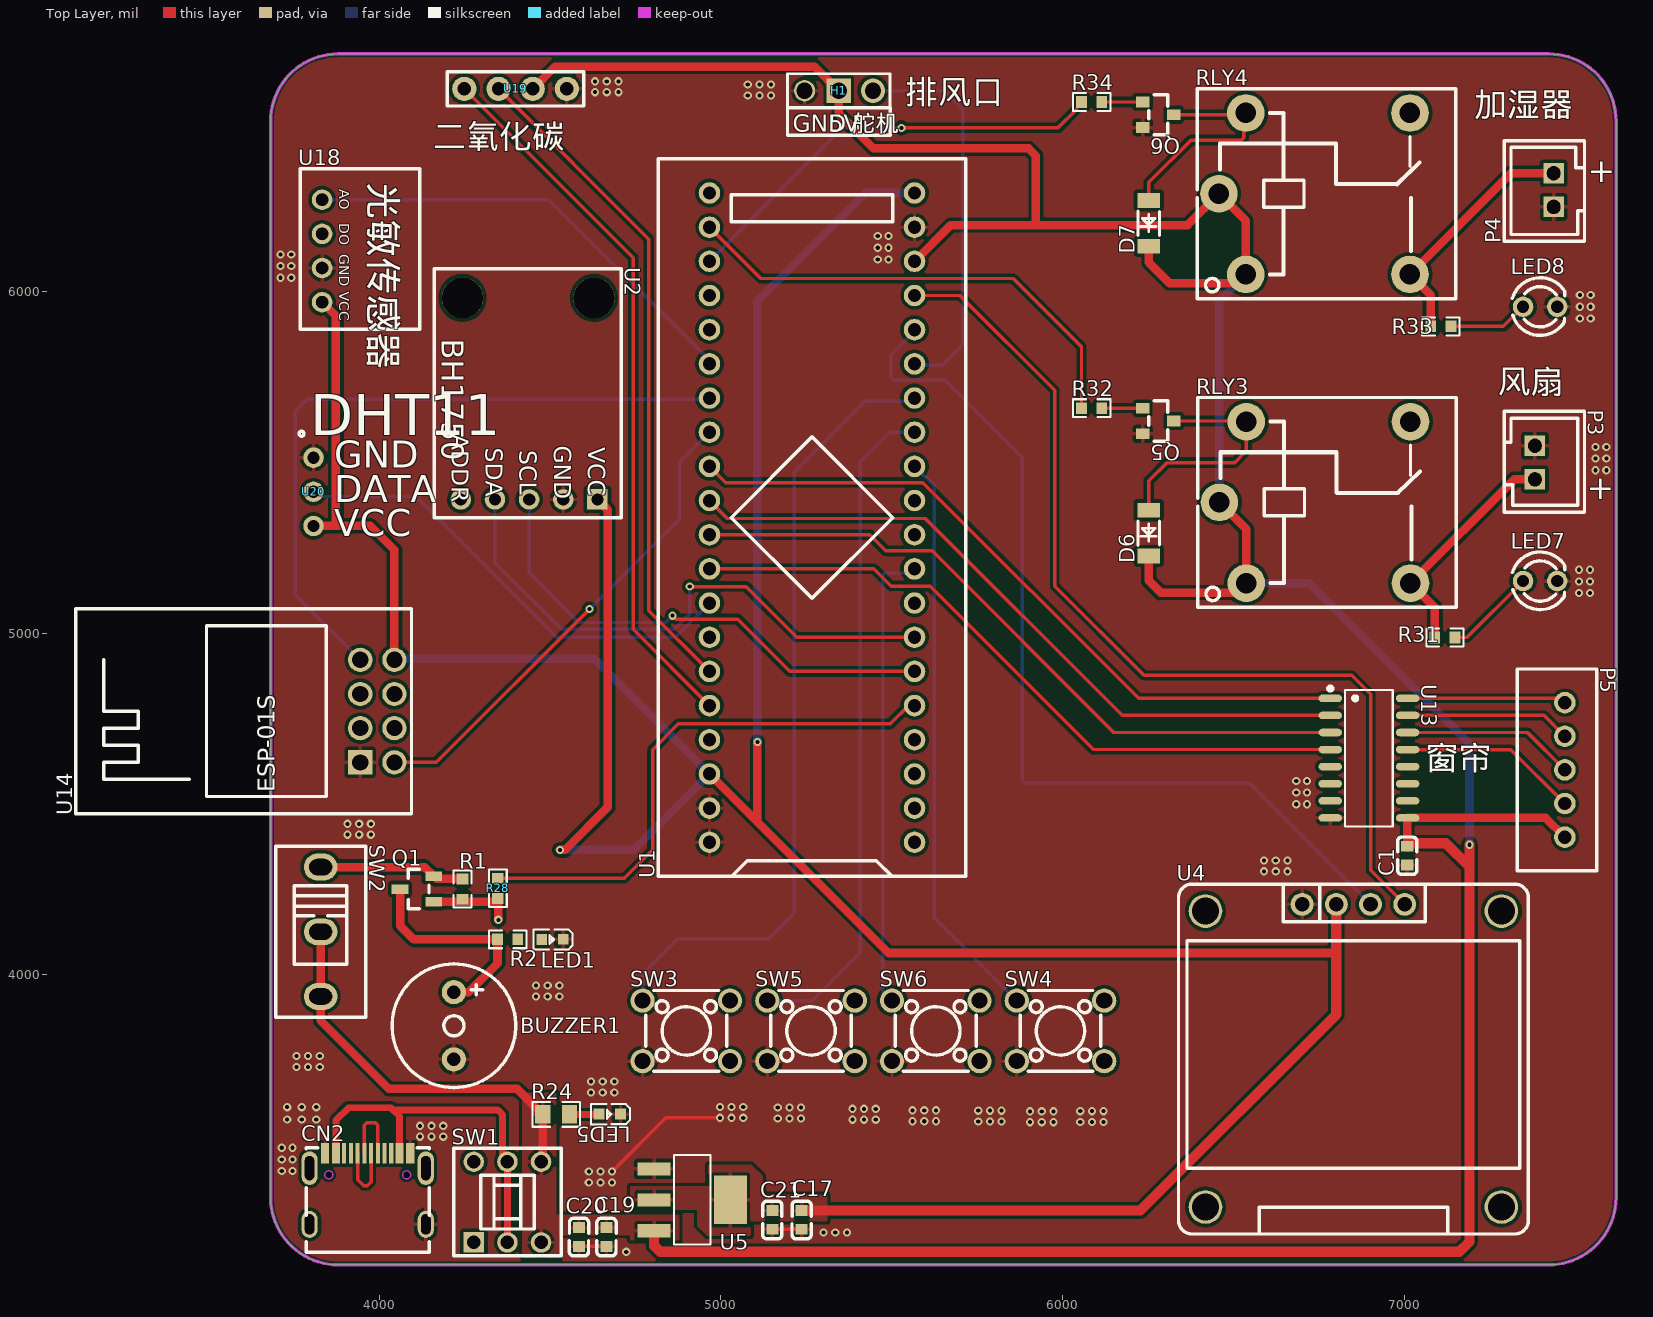
[diagram p0: Top Layer view]
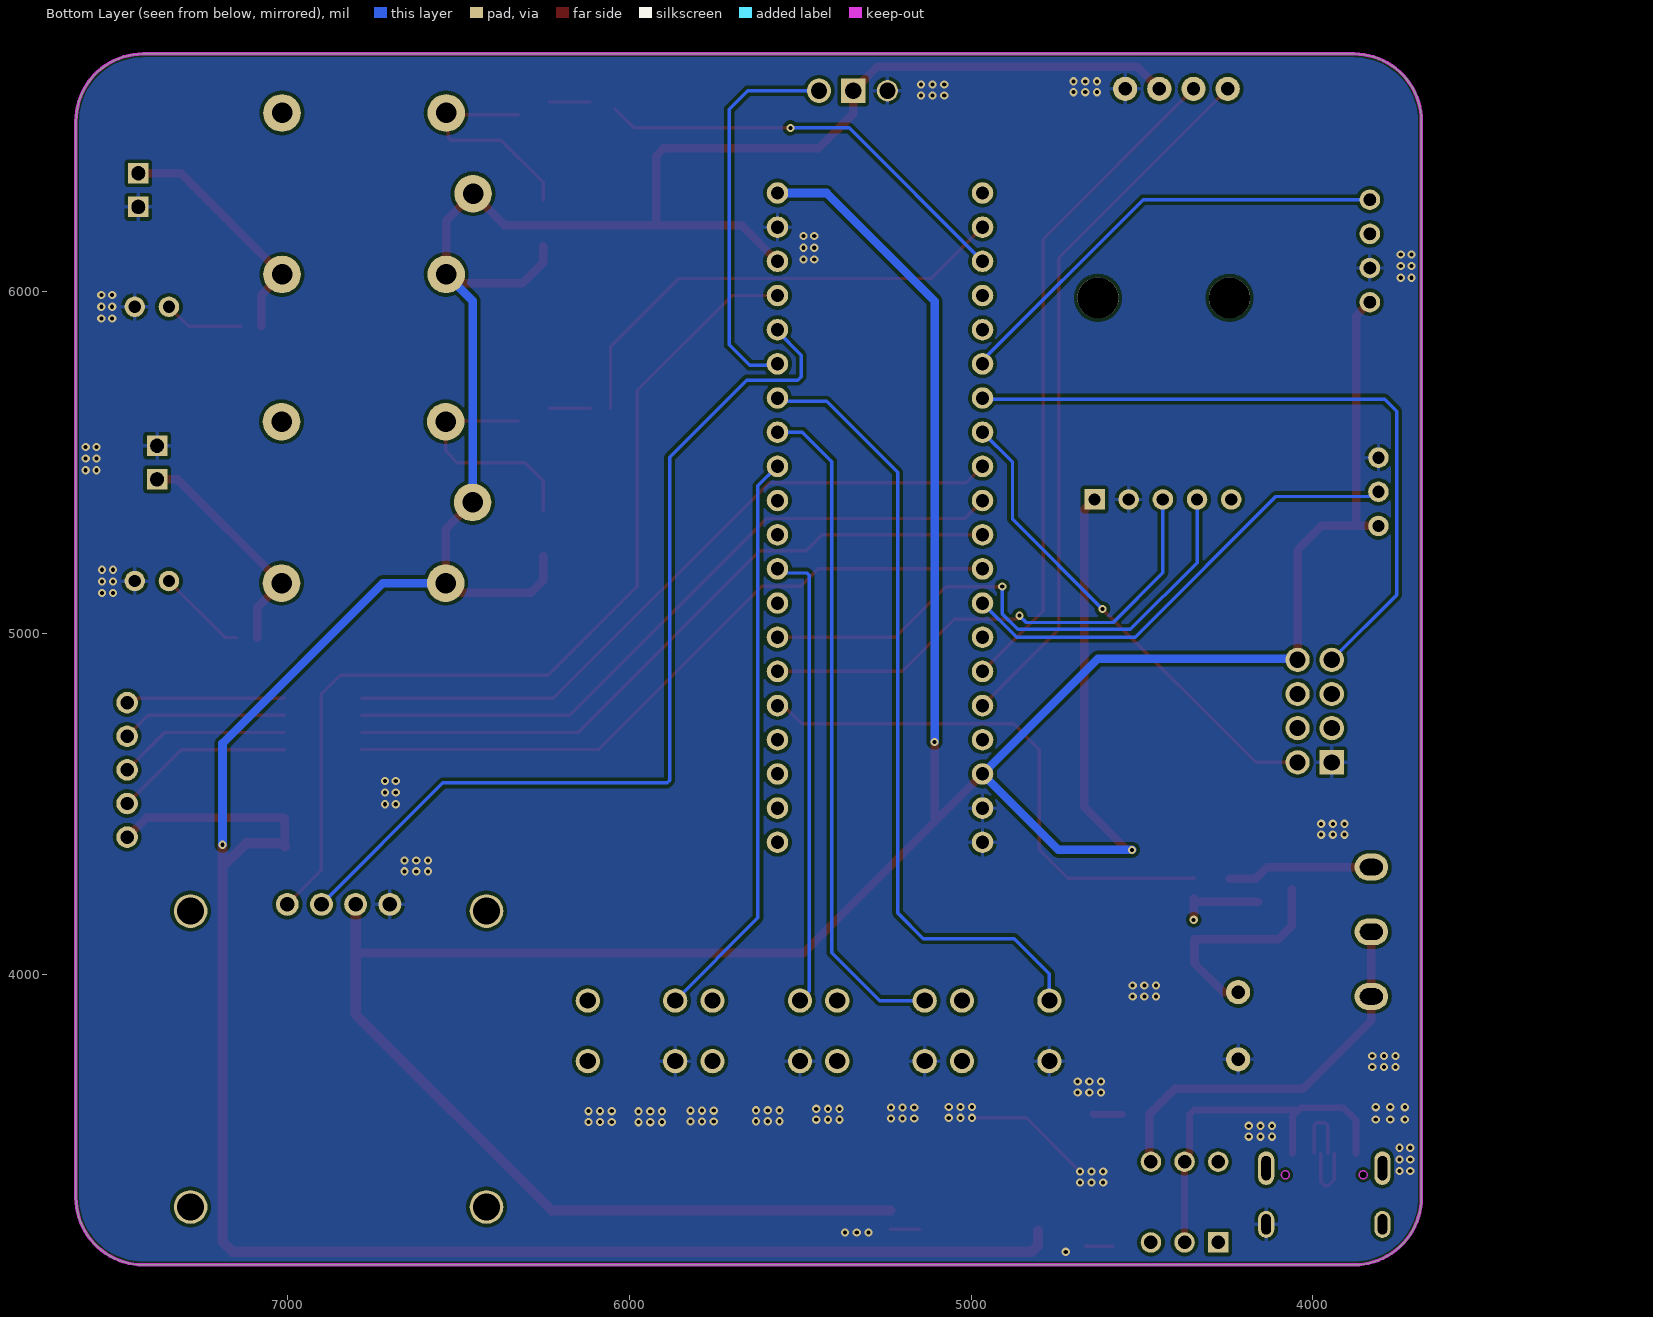
[diagram p1: Bottom Layer view, seen from below]
# Altium PCB MISC51844.pcbdoc
Units mil, origin at the board's own origin, x right, y up, seen from the top; angles counter-clockwise.
Board outline 3937.01 x 3543.31 mil, 2 copper layers (Top Layer, Bottom Layer), stack 62.206 mil thick; 45 components, 47 nets, 206 pads, 156 vias.

## Layer stack, top to bottom
Top Solder Mask Layer: solder mask 0.394, Dk 3.3
Top Layer: signal copper 1.379
Dielectric1: surface 59.449, FR4, Dk 4.5
Bottom Layer: signal copper 1.378
Bottom Solder Mask Layer: solder mask 0.394, Dk 3.3

## Board outline
3879.19,6694.72 ccw(c3879.19,6497.87) 3682.34,6497.87 3682.34,3348.26 ccw(c3879.19,3348.26) 3879.19,3151.41 7422.5,3151.41 ccw(c7422.5,3348.26) 7619.35,3348.26 7619.35,6497.87 ccw(c7422.5,6497.87) 7422.5,6694.72 3879.19,6694.72

## Design rules (kind name [scope] priority, off if disabled: settings)
BoardOutlineClearance copperThickness2oz_1 [All] p2 off: genericclearance=7.99 ignorepadtopadclearanceinfootprint=FALSE except(0: Arc-SplitContinuation Track-SplitContinuation SMDPad-SplitContinuation THPad-SplitContinuation Via-SplitContinuation Fill-SplitContinuation Region-SplitContinuation Poly-SplitContinuation Text-SplitContinuation Hole-SplitContinuation; 5.98: Arc-CutoutEdge SMDPad-CutoutEdge THPad-CutoutEdge Via-CutoutEdge Fill-CutoutEdge Region-CutoutEdge Text-CutoutEdge; 6.93: Hole-OutlineEdge Hole-CutoutEdge; 10: Poly-OutlineEdge Poly-CutoutEdge; 11.81: Arc-OutlineEdge Track-OutlineEdge SMDPad-OutlineEdge THPad-OutlineEdge Via-OutlineEdge Fill-OutlineEdge Region-OutlineEdge Text-OutlineEdge Track-CutoutEdge)
BoardOutlineClearance copperThickness1oz_1 [All] p4: genericclearance=4.02 ignorepadtopadclearanceinfootprint=FALSE except(0: Arc-SplitContinuation Track-SplitContinuation SMDPad-SplitContinuation THPad-SplitContinuation Via-SplitContinuation Fill-SplitContinuation Region-SplitContinuation Poly-SplitContinuation Text-SplitContinuation Hole-SplitContinuation; 6: SMDPad-CutoutEdge THPad-CutoutEdge Via-CutoutEdge Fill-CutoutEdge Region-CutoutEdge Text-CutoutEdge; 6.93: Hole-OutlineEdge Hole-CutoutEdge; 10: Poly-OutlineEdge Poly-CutoutEdge; 11.8: Arc-OutlineEdge Track-OutlineEdge SMDPad-OutlineEdge THPad-OutlineEdge Via-OutlineEdge Fill-OutlineEdge Region-OutlineEdge Text-OutlineEdge; 11.81: Arc-CutoutEdge Track-CutoutEdge)
Clearance copperThickness2oz [All] p1 off: gap=7.99 ignorepadtopadclearanceinfootprint=FALSE except(5.98: SMDPad-Track SMDPad-SMDPad THPad-Track SMDPad-THPad THPad-THPad Track-Via SMDPad-Via THPad-Via Via-Via Fill-Track Region-Track Fill-SMDPad Region-SMDPad Fill-THPad Region-THPad Fill-Via Region-Via Fill-Fill Fill-Region Region-Region Arc-Track Arc-SMDPad Arc-THPad Arc-Via Fill-Arc Region-Arc Arc-Arc Text-Track SMDPad-Text Text-THPad Text-Via Fill-Text Region-Text Arc-Text Text-Text; 6.93: Hole-Track Hole-SMDPad Hole-THPad Hole-Via Fill-Hole Region-Hole Hole-Arc Hole-Text; 10: Poly-Track Poly-SMDPad Poly-THPad Poly-Via Poly-Fill Poly-Region Poly-Poly Poly-Arc Poly-Text Poly-Hole)
Clearance copperThickness1oz [All] p3: gap=4.02 ignorepadtopadclearanceinfootprint=FALSE except(5.98: SMDPad-Track SMDPad-SMDPad THPad-Track SMDPad-THPad THPad-THPad Track-Via SMDPad-Via THPad-Via Via-Via Fill-Track Region-Track Fill-SMDPad Region-SMDPad Fill-THPad Region-THPad Fill-Via Region-Via Fill-Fill Fill-Region Region-Region; 6: Arc-Track Arc-SMDPad Arc-THPad Arc-Via Fill-Arc Region-Arc Arc-Arc Text-Track SMDPad-Text Text-THPad Text-Via Fill-Text Region-Text Arc-Text Text-Text; 6.93: Hole-Track Hole-SMDPad Hole-THPad Hole-Via Fill-Hole Region-Hole Hole-Arc Hole-Text; 10: Poly-Track Poly-SMDPad Poly-THPad Poly-Via Poly-Fill Poly-Region Poly-Poly Poly-Arc Poly-Text Poly-Hole)
DiffPairsRouting differentialPair [All] p1: maxlimit=6 minlimit=6 mostfreqgap=6 toplayer_minwidth=5 toplayer_prefwidth=10 toplayer_maxwidth=100 toplayer_mingap=6 toplayer_prefgap=6 toplayer_maxgap=6 bottomlayer_minwidth=5 bottomlayer_prefwidth=10 bottomlayer_maxwidth=100 bottomlayer_mingap=6 bottomlayer_prefgap=6 bottomlayer_maxgap=6 maxuncoupledlength=10
HoleToHoleClearance otherClearance [All] p1: gap=11.81 allowstackedmicrovias=TRUE
Length netLength [All] p1: minlimit=0 maxlimit=0
MatchedLengths netLengthTolerance [All] p1: tolerance=1000
PasteMaskExpansion pasteMaskExpansion [All] p1: expansion=0
PlaneConnect innerPlane [All] p1: planeconnectstyle=Relief reliefexpansion=20 reliefentries=4 reliefconductorwidth=10 reliefairgap=10
PolygonConnect copperRegion [All] p1: connectstyle=Relief reliefconductorwidth=10 reliefentries=4 polygonreliefangle="90 Angle" airgapwidth=10 via.connectstyle=Relief via.reliefconductorwidth=10 via.reliefentries=4 via.polygonreliefangle="90 Angle" via.airgapwidth=10
RoutingVias viaSize [All] p1: holewidth=12.01 width=24.02 viastyle="Through Hole" minholewidth=11.81 minwidth=19.68 maxholewidth=248.03 maxwidth=393.7
SolderMaskExpansion solderMaskExpansion [IsVia] p1: expansion=-1000 istentingtop=TRUE
SolderMaskExpansion solderMaskExpansion [All] p2: expansion=2 istentingtop=FALSE
Width copperThickness2oz_2 [All] p1 off: maxlimit=100 minlimit=8 preferedwidth=10
Width copperThickness1oz_2 [All] p2: maxlimit=100 minlimit=5 preferedwidth=10

## Components (designator, comment, footprint, x,y, rotation, side; value= is the part's Value field where it differs from the comment)
BUZZER1 "HNB09A03" BUZ-TH_BD9.0-P5.00-D0.6-FD 4218.56,3850.88 r270 top
C1 "47pf" C0603#1 7008.29,4348.46 r90 top
C17 "100n" C0603#2 5236.12,3282.62 r90 top
C19 "100n" C0603#2 4665.04,3232.75 r90 top
C20 "10u" C0603#2 4584.63,3232.75 r90 top
C21 "22u" C0603#2 5150.42,3282.62 r90 top
CN2 "USB-TYPEC" USB-C-SMD_MC-307 3966.22,3373.55 r0 top
D6 "LL4148" LL-34_L3.5-W1.5-RD 6251.77,5292.56 r90 top
D7 "LL4148" LL-34_L3.5-W1.5-RD 6251.77,6198.97 r90 top
H1 "舵机模块" 舵机模块 5344.81,6586.97 r0 top
LED1 "" LED_0603 4504.75,4103.27 r180 top
LED5 "" LED_0603 4672.56,3592.05 r180 top
LED7 "" LED_TH-3mm 7397.24,5152.23 r0 top
LED8 "" LED_TH-3mm 7397.24,5954.86 r0 top
P3 "XH2.54直插座-2P" CONN-TH_XH2.54-2P 7381.88,5498.97 r270 top
P4 "XH2.54直插座-2P" CONN-TH_XH2.54-2P 7436.88,6296.23 r90 top
P5 "" CONN-TH_XH2.54-5P 7469.51,4599.63 r270 top
Q1 "" S8550P_SOT 4108.56,4250.88 r0 top
Q5 "" S8050_SOT-23 6279.53,5625.55 r180 top
Q6 "" S8050_SOT-23 6279.53,6521.7 r180 top
R1 "10k" R0603 4243.56,4250.88 r270 top
R2 "1k" R0603 4375.75,4103.67 r180 top
R24 "4.7k" R0805 4517.71,3591.37 r0 top
R28 "1k" R0603 4347.14,4252.97 r270 top
R31 "3.3k" R0603 7118.6,4987.04 r0 top
R32 "1k" R0603 6084.73,5658.26 r0 top
R33 "3.3k" R0603 7106.6,5897.3 r0 top
R34 "1k" R0603 6084.73,6554.14 r0 top
RLY3 "SRD-05VDC-SL-C" RELAY-TH_SRD-XXVDC-XL-C 6738.22,5382.36 r0 top
RLY4 "SRD-05VDC-SL-C" RELAY-TH_SRD-XXVDC-XL-C 6736.75,6285.76 r0 top
SW1 "K8-8081D-NNW" SW-TH_6P-L8.0-W8.0-P2.50 4375.18,3334.76 r0 top
SW2 "XY-SS12D10L3" SW-TH_3P-L12.7-W6.7_XY-SS12D10LXX 3828.56,4125.88 r270 top
SW3 "" SW-TH_4P-L6.0-W6.0-P4.50-LS6.5 4898.56,3835.88 r0 top
SW4 "" SW-TH_4P-L6.0-W6.0-P4.50-LS6.5 5993.56,3835.88 r0 top
SW5 "" SW-TH_4P-L6.0-W6.0-P4.50-LS6.5 5263.56,3835.88 r0 top
SW6 "" SW-TH_4P-L6.0-W6.0-P4.50-LS6.5 5628.56,3835.88 r0 top
U1 "LCKFB-DKX-STM32F103C8T6" CONN-TH_L53.3-W22.9_STM32F103C8T6-CARD 5266.4,5337.77 r90 top
U2 "" BH1750光照传感器 4428.56,5650.88 r270 top
U4 "" OLED_I2C_0.96 6850.79,3753.38 r0 top
U5 "TLV1117LV33DCYT" SOT-223-4_L6.5-W3.5-P2.30-LS7.0-BR 4915.99,3341.32 r180 top
U13 "ULN2003A" SOP-16_L10.0-W3.9-P1.27-LS6.0-BL 6896.1,4634.02 r270 top
U14 "ESP-01S" WIFIM-TH_ESP-01S 3994.43,4771.7 r90 top
U18 "光照强度模块" 光敏传感器 3858.32,6133.69 r0 top
U19 "" 4P排母 4599.05,6642.46 r180 top
U20 "" dht11温湿度传感器 3807.68,5513.39 r0 top

## Footprints (in the part's own frame and the unit in brackets; to place one, negate y for a bottom-side part, rotate by r counter-clockwise, add the part's x,y. Pads: shape width x height; smd on the part's side, far side on the other; paste and mask are expansions set on the pad)
4P排母 [mm]
  round 1.8 hole 1: 1(1.27,1.27) 2(3.81,1.27) 3(6.35,1.27) 4(8.89,1.27)
  silkscreen extent 0,0 10.16,2.54
BH1750光照传感器 [mil]
  rect 60x60 hole 36: 1(260,210)
  round 60 hole 36: 2(260,110) 3(260,10) 4(260,-90) 5(260,-190)
  round 120 hole 120 unplated: ""(-330,200) ""(-330,-185)
  silkscreen extent -415,-267 313,280
BUZ-TH_BD9.0-P5.00-D0.6-FD [mm]
  round 1.8 hole 1 copper offset 0,0 paste+0 mask+0.051: 1(-2.5,0) 2(2.5,0)
  silkscreen extent -4.6,-4.6 4.6,4.6
C0603#1 [mm]
  rect 0.8x0.9 smd: 1(-0.7,0) 2(0.7,0)
  silkscreen extent -1.39,-0.71 1.39,0.71
C0603#2 [mm]
  rect 0.8x0.9 smd paste+0 mask+0.051: 1(-0.7,0) 2(0.7,0)
  silkscreen extent -1.41,-0.71 1.39,0.72
CONN-TH_L53.3-W22.9_STM32F103C8T6-CARD [mm]
  round 1.6 hole 1: 1(-24.13,-7.62) 2(-21.59,-7.62) 3(-19.05,-7.62) 4(-16.51,-7.62) 5(-13.97,-7.62) 6(-11.43,-7.62) 7(-8.89,-7.62) 8(-6.35,-7.62) 9(-3.81,-7.62) 10(-1.27,-7.62) 11(1.27,-7.62) 12(3.81,-7.62) 13(6.35,-7.62) 14(8.89,-7.62) 15(11.43,-7.62) 16(13.97,-7.62) 17(16.51,-7.62) 18(19.05,-7.62) 19(21.59,-7.62) 20(24.13,-7.62) 21(24.13,7.62) 22(21.59,7.62) 23(19.05,7.62) 24(16.51,7.62) 25(13.97,7.62) 26(11.43,7.62) 27(8.89,7.62) 28(6.35,7.62) 29(3.81,7.62) 30(1.27,7.62) 31(-1.27,7.62) 32(-3.81,7.62) 33(-6.35,7.62) 34(-8.89,7.62) 35(-11.43,7.62) 36(-13.97,7.62) 37(-16.51,7.62) 38(-19.05,7.62) 39(-21.59,7.62) 40(-24.13,7.62)
  silkscreen extent -26.67,-11.43 26.67,11.43
CONN-TH_XH2.54-2P [mil]
  rect 60x60 hole 39.37 slot 41.34 at 0 deg paste+0 mask+1.97: 1(-49.21,0) 2(49.21,0)
  silkscreen extent -150,-90 145,145
CONN-TH_XH2.54-5P [mm]
  round 1.6 hole 1 paste+0 mask+0.05: 1(-5,0) 2(-2.5,0) 3(0,0) 4(2.5,0) 5(5,0)
  silkscreen extent -7.5,-3.53 7.5,2.38
dht11温湿度传感器 [mil]
  round 60 hole 36: 1(0,0) 2(0,-100) 3(0,-200)
  silkscreen extent -42,63 -28,77
LED_0603 [mil]
  rect 31.5x31.5 smd paste+0 mask+2: 1(-33.5,-0.4) 2(29.5,-0.2)
  silkscreen extent -61,-30 53,30
LED_TH-3mm [mil]
  round 60 hole 36 paste+0 mask+2: 1(-50,0) 2(50,0)
  silkscreen extent -81,-84 72,85
LL-34_L3.5-W1.5-RD [mm]
  rect 1.1x1.7 smd paste+0 mask+0.051: 1(-1.7,0) 2(1.7,0)
  silkscreen extent -0.9,-0.8 0.9,0.8
OLED_I2C_0.96 [mm]
  round 1.7 hole 1.1: 1(-3.81,11.5) 2(-1.27,11.5) 3(1.27,11.5) 4(3.81,11.5)
  round 2.5 hole 2: 5(-11,11) 6(11,11) 7(11,-11) 8(-11,-11)
  silkscreen extent -13,-13 13,13
R0603 [mil]
  rect 31.75x34.02 smd paste-3937.01 mask+2: 1(-29.65,0) 2(29.66,0)
  silkscreen extent -55,-26 55,26
R0805 [mm]
  rect 1.133x1.377 smd paste-100 mask+0.051: 1(-1,0) 2(1,0)
  silkscreen extent -1.76,-0.92 1.76,0.92
RELAY-TH_SRD-XXVDC-XL-C [mil]
  round 110 hole 60: 1(-200.79,-236.22) 2(279.53,-236.2) 3(279.53,236.2) 4(-200.79,236.22) 5(-279.53,0)
  silkscreen extent -342,-307 413,307
S8050_SOT-23 [mm]
  rect 1x0.8 smd paste+0 mask+0.051: 1(1.15,-0.823) 2(1.15,1.077) 3(-1.15,0.127)
  silkscreen extent -0.7,-1.37 0.7,1.63
S8550P_SOT [mil]
  rect 49.2x27.6 smd paste+0 mask+2: 1(50.84,-37.4) 2(50.84,37.4) 3(-47.56,0)
  silkscreen extent -24,-58 37,58
SOP-16_L10.0-W3.9-P1.27-LS6.0-BL [mm]
  oval 0.56x1.745 smd: 1(-4.445,-2.872) 2(-3.175,-2.872) 3(-1.905,-2.872) 4(-0.635,-2.872) 5(0.635,-2.872) 6(1.905,-2.872) 7(3.175,-2.872) 8(4.445,-2.872) 9(4.445,2.872) 10(3.175,2.872) 11(1.905,2.872) 12(0.635,2.872) 13(-0.635,2.872) 14(-1.905,2.872) 15(-3.175,2.872) 16(-4.445,2.872)
  silkscreen extent -5.33,-3.02 5.08,1.77
SOT-223-4_L6.5-W3.5-P2.30-LS7.0-BR [mm]
  rect 2.47x0.98 smd paste+0 mask+0.051: 1(2.835,-2.3) 2(2.835,0) 3(2.835,2.3)
  rect 2.47x3.6 smd paste+0 mask+0.051: 4(-2.835,0)
  silkscreen extent -1.37,-3.33 1.37,3.33
SW-TH_3P-L12.7-W6.7_XY-SS12D10LXX [mm]
  oval 2x2.5 hole 1.2 slot 1.7 at 90 deg: 1(-4.81,0) 2(0,0) 3(4.81,0)
  silkscreen extent -6.35,-3.35 6.35,3.35
SW-TH_4P-L6.0-W6.0-P4.50-LS6.5 [mm]
  round 1.8 hole 1.2: 1(-3.25,2.25) 2(3.25,2.25) 3(-3.25,-2.25) 4(3.25,-2.25)
  silkscreen extent -3,-3 3,3
SW-TH_6P-L8.0-W8.0-P2.50 [mil]
  rect 60x60 hole 39.37 paste+0 mask+2: 1(-98.43,-118.11)
  round 60 hole 39.37 paste+0 mask+2: 2(0,-118.11) 3(98.42,-118.11) 4(-98.43,118.11) 5(0,118.11) 6(98.42,118.11)
  silkscreen extent -157,-157 157,157
USB-C-SMD_MC-307 [mm]
  oval 1.2x2 hole 0.7 slot 1.5 at 90 deg paste+0 mask+0.051: 0(4.32,-2.64) 1(-4.32,-2.64)
  oval 1.2x2.5 hole 0.7 slot 1.8 at 90 deg paste+0 mask+0.051: 2(4.32,1.54) 3(-4.32,1.54)
  rect 0.6x1.524 smd paste-100 mask+0.051: A1B12(-3.165,2.64) A4B9(-2.365,2.64) B1A12(3.165,2.64) B4A9(2.365,2.64)
  rect 0.3x1.524 smd paste-100 mask+0.051: A5(-1.25,2.64) A6(-0.25,2.64) A7(0.25,2.64) A8(1.25,2.64) B5(1.75,2.64) B6(0.75,2.64) B7(-0.75,2.64) B8(-1.75,2.64)
  Board Outline Layer circle w0.003: c-2.89,1.04 r0.3
  Board Outline Layer circle w0.003: c2.89,1.04 r0.3
  Board Outline Layer region: -2.59,1.04 -2.62,0.91 -2.703,0.806 -2.823,0.748 -2.957,0.748 -3.077,0.806 -3.16,0.91 -3.19,1.04 -3.19,1.04 -3.16,1.17 -3.077,1.275 -2.957,1.333 -2.823,1.333 -2.703,1.275 -2.62,1.17 -2.59,1.04
  Board Outline Layer region: -2.59,1.04 -2.599,0.968 -2.624,0.901 -2.665,0.841 -2.72,0.793 -2.784,0.76 -2.854,0.742 -2.926,0.742 -2.996,0.76 -3.06,0.793 -3.115,0.841 -3.156,0.901 -3.181,0.968 -3.19,1.04 -3.181,1.112 -3.156,1.18 -3.115,1.239 -3.06,1.287 -2.996,1.321 -2.926,1.338 -2.854,1.338 -2.784,1.321 -2.72,1.287 -2.665,1.239 -2.624,1.18 -2.599,1.112
  Board Outline Layer region: 3.19,1.04 3.16,0.91 3.077,0.806 2.957,0.748 2.823,0.748 2.703,0.806 2.62,0.91 2.59,1.04 2.59,1.04 2.62,1.17 2.703,1.275 2.823,1.333 2.957,1.333 3.077,1.275 3.16,1.17 3.19,1.04
  Board Outline Layer region: 3.19,1.04 3.181,0.968 3.156,0.901 3.115,0.841 3.06,0.793 2.996,0.76 2.926,0.742 2.854,0.742 2.784,0.76 2.72,0.793 2.665,0.841 2.624,0.901 2.599,0.968 2.59,1.04 2.599,1.112 2.624,1.18 2.665,1.239 2.72,1.287 2.784,1.321 2.854,1.338 2.926,1.338 2.996,1.321 3.06,1.287 3.115,1.239 3.156,1.18 3.181,1.112
  Multi-Layer board cut-out: -2.59,1.04 -2.62,0.91 -2.703,0.806 -2.823,0.748 -2.957,0.748 -3.077,0.806 -3.16,0.91 -3.19,1.04 -3.19,1.04 -3.16,1.17 -3.077,1.275 -2.957,1.333 -2.823,1.333 -2.703,1.275 -2.62,1.17 -2.59,1.04
  Multi-Layer board cut-out: 3.19,1.04 3.16,0.91 3.077,0.806 2.957,0.748 2.823,0.748 2.703,0.806 2.62,0.91 2.59,1.04 2.59,1.04 2.62,1.17 2.703,1.275 2.823,1.333 2.957,1.333 3.077,1.275 3.16,1.17 3.19,1.04
  silkscreen extent -4.57,-4.7 4.57,3.05
WIFIM-TH_ESP-01S [mm]
  rect 1.8x1.8 hole 1.2: 1(-3.81,1.27)
  round 1.8 hole 1.2: 2(-1.27,1.27) 3(1.27,1.27) 4(3.81,1.27) 5(3.81,-1.27) 6(1.27,-1.27) 7(-1.27,-1.27) 8(-3.81,-1.27)
  silkscreen extent -7.62,-2.54 7.62,22.4
光敏传感器 [mil]
  round 60 hole 36 slot 36.2 at 90 deg: 1(-25.45,-165.45) 2(-25.45,-65.45) 3(-25.45,34.55) 4(-25.45,134.55)
  silkscreen extent -90,-245 260,225
舵机模块 [mm]
  round 1.575 hole 1.2 paste+0 mask+0.051: 1(-2.54,0)
  rect 1.8x1.8 hole 1.2 paste+0 mask+0.051: 2(0,0)
  round 1.8 hole 1.2 paste+0 mask+0.051: 3(2.54,0)
  silkscreen extent -3.81,-3.3 3.81,1.27

## Via types
v1: diameter 24.02, hole 12, Top Layer to Bottom Layer, 156 vias

## Nets (pads, with @x,y where several pads share a name; then routed paths per layer and width w, separated by ;. In a path a pad name is that pad's centre, name@x,y a point inside that pad or via, vN(x,y) a via of type N, cw(c..) or ccw(c..) an arc to the next point about the centre after c; other vN are vias at no path point)
$1N12: P5.4 U13.13 | length 525.7
  Top Layer w10: U13.13 7311.7,4659.02 P5.4
$1N13: P5.3 U13.14 | length 505.6
  Top Layer w10: U13.14 7360.13,4709.02 P5.3
$1N14: P5.2 U13.15 | length 485.6
  Top Layer w10: U13.15 7408.56,4759.02 P5.2
$1N15: P5.1 U13.16 | length 465.5
  Top Layer w10: U13.16 7456.98,4809.02 P5.1
$1N25: Q6.1 R34.2 | length 119.8
  Top Layer w10: R34.2 Q6.1
$1N27: D7.2 Q6.3 RLY4.4 | length 666
  Top Layer w10: D7.2 6251.77,6318.76 6375.46,6442.44 6522.88,6442.44 6529.95,6449.51 6529.95,6515.97 RLY4.4@6530.68,6516.7 ; Q6.3 RLY4.4@6530.68,6516.7 ; RLY4.4 RLY4.4@6530.68,6516.7
$1N29: P4.2 R33.1 RLY4.2 | length 720.6
  Top Layer w25: R33.1 7076.94,5988.89 RLY4.2 7312.17,6345.45 P4.2
$1N33: LED8.1 R33.2 | length 234.8
  Top Layer w10: R33.2 7289.68,5897.3 LED8.1
$1N35: Q5.1 R32.2 | length 120
  Top Layer w10: R32.2 6233.94,5658.26 Q5.1
$1N37: D6.2 Q5.3 RLY3.4 | length 706.6
  Top Layer w10: D6.2 6251.77,5445.42 6305.24,5498.88 6502.91,5498.88 6537.43,5533.39 RLY3.4 6535.46,5620.54 Q5.3
$1N39: P3.2 R31.1 RLY3.2 | length 678.5
  Top Layer w25: R31.1 7088.94,5074.97 RLY3.2 7321.34,5449.75 P3.2
$1N43: LED7.1 R31.2 | length 267.4
  Top Layer w10: R31.2 7182.05,4987.04 LED7.1
$1N57: LED5.2 R24.2 | length 86.3
  Top Layer w20: R24.2 4642.18,3591.37 LED5.2
$1N74: BUZZER1.1 Q1.3 R2.2 | length 641.6
  Top Layer w25: Q1.3 4061,4143.44 4100.77,4103.67 R2.2 4346.09,4033.41 4261.98,3949.3 BUZZER1.1
$1N76: Q1.1 R1.2 R28.2 | length 254.8
  Top Layer w25: Q1.1 4337.3,4213.48 R28.2 4348.56,4221.89 v1(4348.56,4160.88)
$1N136: Q1.2 R1.1 SW2.1 | length 429.4
  Top Layer w25: SW2.1@3828.56,4315.25 4132.43,4315.25 Q1.2 4167.14,4280.53 R1.1
$1N137: LED1.2 R2.1
+5V: C1.2 C19.2 C20.2 D6.1 D7.1 H1.2 P5.5 R24.1 RLY3.1 RLY3.5 RLY4.1 RLY4.5 SW1.3 SW1.6 SW2.2 SW2.3 U1.18 U5.3 U13.9 U19.2 | length 11515.4
  Top Layer w25: SW2.2 SW2.3 3828.56,3865.88 4028.56,3665.88 4403.83,3665.88 R24.1 4478.34,3457.61 SW1.6 ; U19.2 4514.41,6657.82 5273.96,6657.82 H1.2 5344.81,6519.46 5446,6418.26 5899.98,6418.26 5921.76,6396.49 5921.76,6202.16 5913.38,6193.79 ; U1.18 5672.42,6193.79 5913.38,6193.79 ; D6.1 6251.77,5153.37 6287.23,5117.91 6509.2,5117.91 RLY3.1 6537.43,5303.62 RLY3.5 ; D7.1 6251.77,6084.78 6312.92,6023.64 6510.06,6023.64 RLY4.1 6535.96,6207.02 RLY4.5 6365.25,6193.79 5913.38,6193.79 ; C1.2 7008.29,4458.12 U13.9 7413.28,4459.02 P5.5
  Top Layer w30: U5.3 4804.38,3207.06 4822.07,3189.37 7161.03,3189.37 7190.44,3218.78 7190.44,4315.67 ; C1.2 7017.17,4384.91 7121.19,4384.91 7190.44,4315.67 ; v1(7190.44,4380.4) 7190.44,4315.67
  Bottom Layer w25: RLY3.5 6458.69,5972.27 RLY4.1 ; RLY3.1 6721.22,5146.14 7190.44,4676.92 v1(7190.44,4380.4)
BEEP: R28.1 U1.5 | length 1582.6
  Top Layer w10: R28.1 4717.12,4282.62 4800.03,4365.54 4800.03,4658.7 4875.42,4734.08 5495.24,4734.08 U1.5@5548.85,4787.69
ESP_RX: U1.27 U14.4 | length 2033.9
  Bottom Layer w10: U14.4 3754.74,5111.39 3754.74,5649.43 3789.92,5684.61 4963.24,5684.61 U1.27
ESP_TX: U1.28 U14.8 | length 1419.6
  Top Layer w10: U14.8 4166.75,4621.7 v1(4615.28,5070.23)
  Bottom Layer w10: v1(4615.28,5070.23) 4878.56,5333.51 4878.56,5499.93 U1.28
GND: BUZZER1.2 C1.1 C17.1 C19.1 C20.1 C21.1 CN2.0 CN2.A1B12 CN2.B1A12 H1.1 LED1.1 LED5.1 LED7.2 LED8.2 P3.1 P4.1 Q5.2 Q6.2 SW3.3 SW4.3 SW5.3 SW6.3 U1.19 U1.39 U1.40 U2.2 U4.1 U5.1 U13.8 U14.1 U18.2 U19.1 U20.1 | length 546.7
  Top Layer w10: C20.1 C19.1 ; v1(4681.56,3424.27) 4838.76,3581.47 v1(4996.99,3581.47) ; C21.1 C17.1
  other v1: 4722.96,3189.25 5300.28,3246.22 5334.4,3246.22 5368.53,3246.22 4613.31,3392.5 4647.43,3392.5 4681.56,3392.5 4613.31,3424.27 4647.43,3424.27 3714.67,3425.66 3746.43,3425.66 3714.67,3459.78 3746.43,3459.78 3714.67,3493.9 3746.43,3493.9 4119.07,3526.29 4153.2,3526.29 4187.32,3526.29 4119.07,3558.06 4153.2,3558.06 4187.32,3558.06 5904.69,3568.66 5938.82,3568.66 5972.94,3568.66 6051.39,3569.1 6085.52,3569.1 6119.64,3569.1 5752.94,3570.55 5787.07,3570.55 5821.19,3570.55 5560.85,3571.54 5594.98,3571.54 5629.1,3571.54 3730.61,3576.45 3773.14,3576.45 3815.67,3576.45 5384.65,3576.01 5418.77,3576.01 5452.9,3576.01 5166.13,3579.48 5200.25,3579.48 5234.37,3579.48 5031.12,3581.47 5065.24,3581.47 5904.69,3600.43 5938.82,3600.43 5972.94,3600.43 6051.39,3600.87 6085.52,3600.87 6119.64,3600.87 5752.94,3602.32 5787.07,3602.32 5821.19,3602.32 5560.85,3603.31 5594.98,3603.31 5629.1,3603.31 5384.65,3607.78 5418.77,3607.78 5452.9,3607.78 5166.13,3611.25 5200.25,3611.25 5234.37,3611.25 3730.61,3612.59 3773.14,3612.59 3815.67,3612.59 4996.99,3613.24 5031.12,3613.24 5065.24,3613.24 4619.63,3655.76 4653.76,3655.76 4687.88,3655.76 4619.63,3687.53 4653.76,3687.53 4687.88,3687.53 3757.71,3730.18 3791.83,3730.18 3825.95,3730.18 3757.71,3761.94 3791.83,3761.94 3825.95,3761.94 4458.78,3936.79 4492.9,3936.79 4527.03,3936.79 4458.78,3968.55 4492.9,3968.55 4527.03,3968.55 6589.36,4302.73 6623.49,4302.73 6657.61,4302.73 6589.36,4334.49 6623.49,4334.49 6657.61,4334.49 3907.08,4409.97 3941.2,4409.97 3975.33,4409.97 3907.08,4441.74 3941.2,4441.74 3975.33,4441.74 6683.54,4498.97 6715.31,4498.97 6683.54,4533.1 6715.31,4533.1 6683.54,4567.22 6715.31,4567.22 7511.1,5116.94 7542.86,5116.94 7511.1,5151.06 7542.86,5151.06 7511.1,5185.19 7542.86,5185.19 7559.12,5476.55 7590.89,5476.55 7559.12,5510.67 7590.89,5510.67 7559.12,5544.8 7590.89,5544.8 7513.33,5920.73 7545.1,5920.73 7513.33,5954.86 7545.1,5954.86 7513.33,5988.98 7545.1,5988.98 3710.86,6039.88 3742.63,6039.88 3710.86,6074.01 3742.63,6074.01 5458.66,6093.49 5490.43,6093.49 3710.86,6108.13 3742.63,6108.13 5458.66,6127.61 5490.43,6127.61 5458.66,6161.74 5490.43,6161.74 5078.33,6573.22 5112.45,6573.22 5146.57,6573.22 4631.6,6582.77 4665.73,6582.77 4699.85,6582.77 5078.33,6604.99 5112.45,6604.99 5146.57,6604.99 4631.6,6614.54 4665.73,6614.54 4699.85,6614.54
IN1: U1.29 U13.1 | length 2097.8
  Top Layer w10: U1.29 5013.7,5440.48 5590.9,5440.48 6222.35,4809.02 U13.1
IN2: U1.30 U13.2 | length 2077
  Top Layer w10: U1.30 5018.86,5335.31 5597.42,5335.31 6173.7,4759.02 U13.2
IN3: U1.31 U13.3 | length 2056.3
  Top Layer w10: U1.31 5435.18,5287.77 5482.57,5240.38 5617.7,5240.38 6149.06,4709.02 U13.3
IN4: U1.32 U13.4 | length 2035.6
  Top Layer w10: U1.32 5447.67,5187.77 5498.07,5137.38 5611.98,5137.38 6089.97,4659.39 6782.65,4659.39 U13.4
JDQ1: R32.1 U1.22 | length 1412.9
  Top Layer w10: U1.22 5116.68,6037.49 5854.93,6037.49 6055.07,5837.35 R32.1
JDQ2: R34.1 U1.23 | length 1259.3
  Top Layer w10: v1(5528.46,6478.25) 5986.35,6478.25 6041.21,6533.11
  Bottom Layer w10: U1.23 5356.88,6478.25 v1(5528.46,6478.25)
KEY1: SW3.1 U1.14 | length 2327.5
  Bottom Layer w10: SW3.1 4770.61,4002.93 4873.56,4105.88 5139.81,4105.88 5214.81,4180.88 5214.81,5470.35 5422.53,5678.08 5556.7,5678.08 U1.14
KEY2: SW5.1 U1.13 | length 1961.4
  Bottom Layer w10: SW5.1 5267.14,3924.46 5407.46,4064.78 5407.46,5501.62 5493.61,5587.77 U1.13
KEY3: SW4.1 U1.12 | length 1687.3
  Bottom Layer w10: U1.12 5623.56,5430.62 5623.56,4166.51 SW4.1
KEY4: SW6.1 U1.9 | length 1353.4
  Bottom Layer w10: SW6.1 5473.2,3951.86 5473.2,5168.75 5480.27,5175.82 5541.7,5175.82 U1.9@5560.31,5194.44
LED1: U1.1
LED2: U1.2
OLED_SCL: U1.16 U4.3 | length 2763.4
  Bottom Layer w10: U1.16 5566.4,5882.63 5497.08,5813.31 5497.08,5750.4 5507.08,5740.4 5655.98,5740.4 5882.26,5514.12 5882.26,4568.47 5889.33,4561.4 6545.53,4561.4 U4.3
OLED_SDA: U1.17 U4.4 | length 2809.8
  Top Layer w10: U1.17 5699.16,5987.77 5976.59,5710.34 5976.59,5137.42 6237.93,4876.09 6846.03,4876.09 6901.31,4820.81 6901.31,4305.62 U4.4
PA1: U1.26 U18.4 | length 1338.6
  Bottom Layer w10: U18.4 4496.2,6268.24 4966.4,5798.03 U1.26
PB0: U1.33 U20.2 | length 1376.2
  Bottom Layer w10: U20.2 3821.52,5399.55 4108.3,5399.55 4519.84,4988.01 4866.64,4988.01 U1.33
PB7: H1.3 U1.15 | length 1141.9
  Bottom Layer w10: H1.3 5652.87,6586.97 5707.57,6532.28 5707.57,5843.77 5647.26,5783.46 5570.71,5783.46 U1.15
PB10: U1.35 U19.3 | length 1960.4
  Top Layer w10: U19.3 4788.56,6152.95 4788.56,5065.62 U1.35
PB11: U1.36 U19.4 | length 2101.8
  Top Layer w10: U19.4 4743.56,6097.95 4743.56,5010.62 U1.36
SCL: U1.6 U2.3 | length 1478.7
  Top Layer w10: v1(4858.56,5050.88) 4868.56,5040.88 5048.56,5040.88 5201.66,4887.77 U1.6
  Bottom Layer w10: U2.3 4438.56,5175.88 4583.56,5030.88 4838.56,5030.88 v1(4858.56,5050.88)
SDA: U1.7 U2.4 | length 1653.6
  Top Layer w10: v1(4908.56,5135.88) 5073.56,5135.88 5221.66,4987.77 U1.7
  Bottom Layer w10: U2.4 4338.56,5205.88 4533.56,5010.88 4863.56,5010.88 4908.56,5055.88 v1(4908.56,5135.88)
USB_D+: CN2.A6 CN2.B6 | length 210.7
  Top Layer w10: CN2.A6 3956.37,3560 3963.44,3567.07 3989,3567.07 3996.07,3560 3996.07,3477.82 CN2.B6
USB_D-: CN2.A7 CN2.B7 | length 212.2
  Top Layer w10: CN2.B7 3936.69,3400.44 3954.66,3382.47 3964.66,3382.47 3976.06,3393.87 CN2.A7
V_USB: CN2.A4B9 CN2.B4A9 SW1.2 SW1.5 | length 1122.8
  Top Layer w20: CN2.A4B9 3873.11,3574.44 3909.4,3610.73 4034.65,3610.73 4040.74,3604.63 ; CN2.B4A9 4059.33,3586.05 4040.74,3604.63 ; SW1.2 SW1.5 4360.99,3467.07 4360.99,3590.49 4346.84,3604.63 4040.74,3604.63
VCC: C17.2 C21.2 U1.20 U1.38 U2.1 U4.2 U5.2 U5.4 U14.5 U18.1 U20.3 | length 10247.7
  Top Layer w25: U20.3 3873.23,5313.39 ; U18.1 3873.23,5927.87 3873.23,5313.39 ; U14.5 4044.43,5243.09 3974.13,5313.39 3873.23,5313.39 ; v1(4528.65,4365.54) 4543.22,4365.54 4668.56,4490.88 4668.56,5360.88 U2.1 ; U1.38 5106.71,4447.46 ; v1(5106.71,4681.58) 5106.71,4447.46 ; 6800.79,4064.88 6799.7,4063.79 5490.39,4063.79 5106.71,4447.46
  Top Layer w30: C17.2 6227.45,3310.17 6800.79,3883.51 6800.79,4064.88 U4.2
  Bottom Layer w25: U14.5 4048.11,4925.38 4628.8,4925.38 U1.38 4744.17,4365.54 v1(4528.65,4365.54) ; v1(5106.71,4681.58) 5106.71,5971.62 5422.86,6287.77 U1.20
pads on no net: CN2.1 CN2.2 CN2.3 CN2.A5 CN2.A8 CN2.B5 CN2.B8 RLY3.3 RLY4.3 SW1.1 SW1.4 SW3.2 SW3.4 SW4.2 SW4.4 SW5.2 SW5.4 SW6.2 SW6.4 U1.3 U1.4 U1.8 U1.10 U1.11 U1.21 U1.24 U1.25 U1.34 U1.37 U2. U2.5 U4.5 U4.6 U4.7 U4.8 U13.5 U13.6 U13.7 U13.10 U13.11 U13.12 U14.2 U14.3 U14.6 U14.7 U18.3

## Polygon pours and split planes (outlines as drawn)
GND on Bottom Layer (solid, remove dead copper, pour order 6): 3000,7079.23 3000,3000 7927.3,3000 7927.3,7079.23
+5V on Top Layer (solid, remove dead copper, pour order 4): 4413.78,3654.6 4517.71,3654.6 4517.71,3298.16 4878.2,3298.16 4878.2,3222.66 4735.98,3222.66 4734.22,3224.42 4734.22,3238.47 4527.04,3238.47 4527.04,3171.74 4423.71,3171.74 4418.17,3177.28 4418.17,3650.21
VCC on Top Layer (solid, remove dead copper, pour order 6): 4735.25,3381.27 4963.07,3381.27 4963.07,3444.48 5089.49,3444.48 5122.48,3411.49 5122.48,3356.25 5310.72,3356.25 5310.72,3278.56 5086.85,3278.56 5086.85,3236.42 4959.12,3236.42 4930.14,3265.39 4930.14,3312.8 4748.42,3312.8 4733.93,3327.28 4733.93,3379.96
GND on Top Layer (solid, remove dead copper, pour order 8): 3156.78,6738.16 3156.78,3074.48 8134.96,3074.48 8134.96,6738.16

## Keep-outs
Board Outline Layer:
  the board outline again, w10

## Silkscreen, mask and mechanical layers (free items; w line width, h text height)
Top Silkscreen Layer:
  text "排风口" at 5539.73,6524.95 h120
  text "加湿器" at 7205.03,6489.42 h120
  text "二氧化碳" at 4158.15,6394.7 h120
  text "+" at 7535.96,6296.42 h120
  text "风扇" at 7272.87,5679.04 h120
  text "+" at 7533.73,5367.99 h120
  text "窗帘" at 7062.08,4576.41 h120